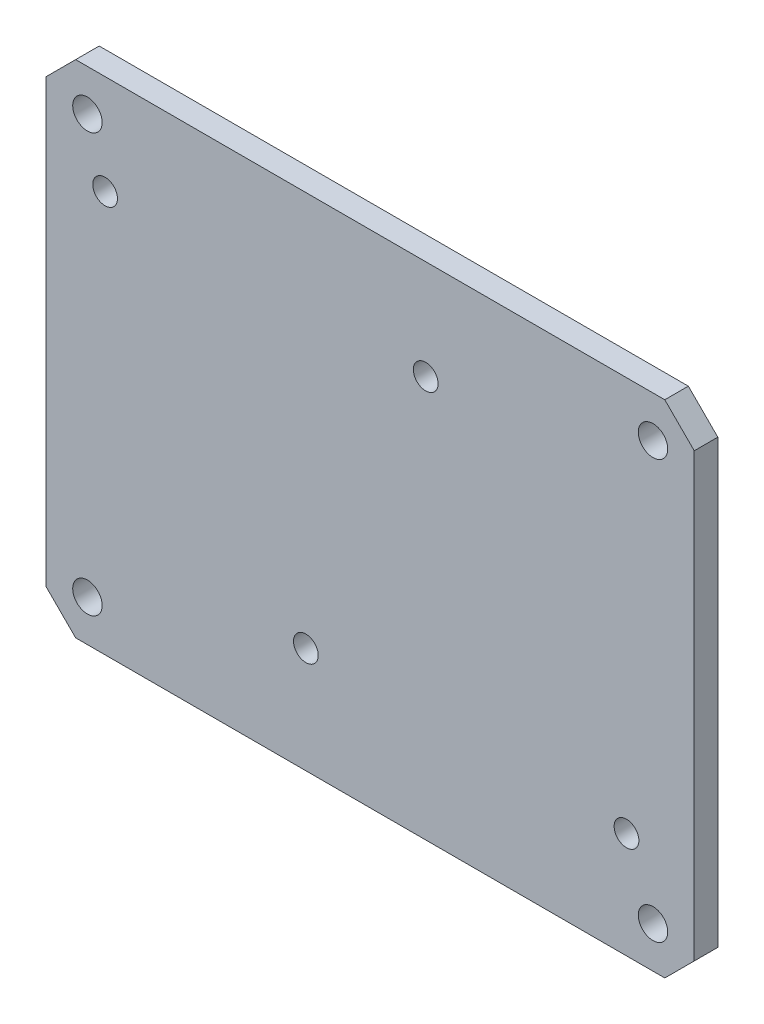
SolidWorks part; units mm, degrees
material "6061-T6 (SS)"
ref_plane "前视基准面" through (0, 0, 0) normal (0, 0, 1) x (1, 0, 0)
ref_plane "上视基准面" through (0, 0, 0) normal (0, 1, 0) x (1, 0, 0)
ref_plane "右视基准面" through (0, 0, 0) normal (1, 0, 0) x (0, 0, -1)
sketch "草图1" plane through (0, 0, 0) normal (0, 0, 1) x (1, 0, 0)
  line L1 (-76.0336, 31.3849) -> (33.9664, 31.3849)
  line L2 (-76.0336, 31.3849) -> (-76.0336, -53.6151)
  line L3 (-76.0336, -53.6151) -> (33.9664, -53.6151)
  line L4 (33.9664, 31.3849) -> (33.9664, -53.6151)
  dimension "D1" = 85
  dimension "D2" = 110
extrude "凸台-拉伸1" add sketch "草图1" along normal blind 4
hole_wizard "M5 螺纹孔1" positions "草图3" profile "草图2" tap size "M5" standard "Gb"
sketch "草图3" plane through (0, 0, 4) normal (0, 0, 1) x (1, 0, 0)
  line L0 (-76.0336, 31.3849) -> (-76.0336, -53.6151) construction
  line L1 (-76.0336, -53.6151) -> (33.9664, -53.6151) construction
  point P0 (-66.0336, 14.4949)
  point P3 (-31.9536, -35.6151)
  point P6 (-11.6136, 14.4949)
  point P9 (22.4664, -35.6151)
  dimension "D1" = 54.42
  dimension "D2" = 50.11
  dimension "D3" = 10
  dimension "D4" = 54.42
  dimension "D5" = 18
sketch "草图2" plane through (-66.0336, 14.4949, 4) normal (1, 0, 0) x (0, -1, 0)
  line L0 (0, 0) -> (0, 17.2618)
  line L1 (0, 17.2618) -> (2.1, 16)
  line L2 (2.1, 16) -> (2.1, 0)
  line L5 (2.1, 0) -> (0, 0)
  line L10 (0, 17.2618) -> (-2.1, 16) construction
  line L11 (0, -6.35) -> (0, 107.95) construction
  dimension "螺纹孔钻头直径" = 4.2
  dimension "螺纹孔钻头深度" = 16
  dimension "导头角度" = 118
cosmetic thread "孔螺蚊线1" parameters "D1"=4, "D2"=5
cosmetic thread "孔螺蚊线2" parameters "D1"=4, "D2"=5
cosmetic thread "孔螺蚊线3" parameters "D1"=4, "D2"=5
cosmetic thread "孔螺蚊线4" parameters "D1"=4, "D2"=5
chamfer "倒角1" distance 5 angle 45 4 edges at (-76.0336, -53.6151, 2) (-76.0336, 31.3849, 2) (33.9664, -53.6151, 2) (33.9664, 31.3849, 2)
hole_wizard "Ø5.0 (5) 直径孔1" positions "草图5" profile "草图4" hole size "Ø5.0" standard "Ansi Metric"
sketch "草图5" plane through (0, 0, 0) normal (0, 0, -1) x (-1, 0, 0)
  point P0 (69.0336, 24.3849)
  point P3 (69.0336, -46.6151)
  point P6 (-26.9664, -46.6151)
  point P9 (-26.9664, 24.3849)
sketch "草图4" plane through (-69.0336, 24.3849, 0) normal (1, 0, 0) x (0, 1, 0)
  line L0 (0, 0) -> (0, 11.4434)
  line L1 (0, 11.4434) -> (2.5, 10)
  line L2 (2.5, 10) -> (2.5, 0)
  line L5 (2.5, 0) -> (0, 0)
  line L10 (0, 11.4434) -> (-2.5, 10) construction
  line L11 (0, -6.35) -> (0, 107.95) construction
  dimension "孔直径" = 5
  dimension "孔深度" = 10
  dimension "导头角度" = 120
